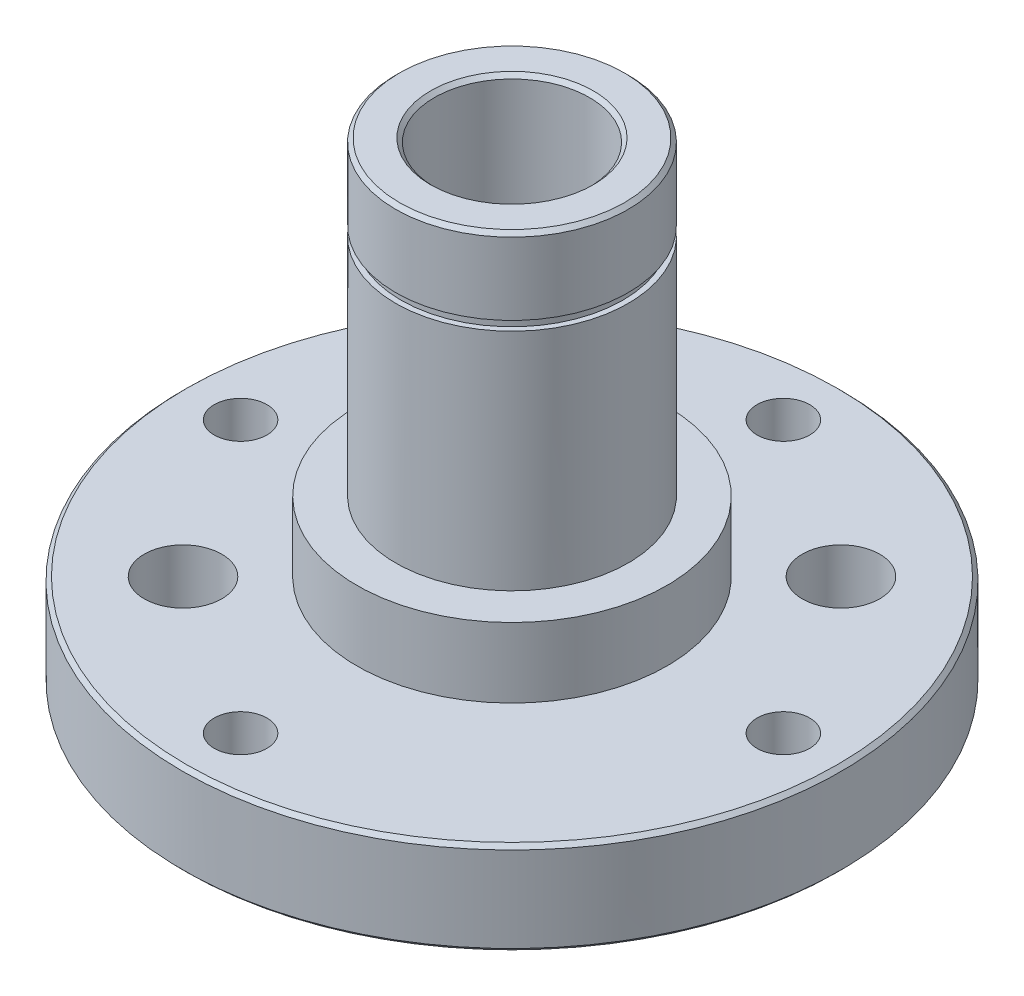
from build123d import *

# Parameters (mm, degrees)
SKETCH2_R                  = 10
CUT_EXTRUDE1_DEPTH         = 86.635856976
SKETCH3_W                  = 0.7
SKETCH3_H                  = 1.2
M8_TAPPED_HOLE1_D          = 6.8
F_10_0_10_DIAMETER_HOLE1_D = 10
CHAMFER1_SIZE              = 0.5


with BuildPart() as part:
    # Sketch1 → Revolve1 (revolve)
    with BuildSketch(Plane.XY, mode=Mode.PRIVATE) as revolve1_sk:
        Polygon((0, 0), (42.5, 0), (42.5, 12), (20, 12), (20, 21), (15, 21), (15, 61), (0, 61), align=None)
    revolve(revolve1_sk.sketch.rotate(Axis((0, 0, 0), (0, 1, 0)), 90), axis=Axis((0, 0, 0), (0, 1, 0)))

    # Sketch2 → Cut-Extrude1 (cut, through all)
    with BuildSketch(Plane(origin=(0, 61, 0), x_dir=(1, 0, 0), z_dir=(0, 1, 0))):
        with Locations(Location((0, 0, 0), (0, 0, 270))):
            Circle(SKETCH2_R)
    extrude(amount=-CUT_EXTRUDE1_DEPTH, mode=Mode.SUBTRACT)

    # Sketch3 → Cut-Revolve1 (revolve, cut)
    with BuildSketch(Plane.XY, mode=Mode.PRIVATE) as cut_revolve1_sk:
        with Locations((14.65, 50.6)):
            Rectangle(SKETCH3_W, SKETCH3_H)
    revolve(cut_revolve1_sk.sketch.rotate(Axis((0, 0, 0), (0, -1, 0)), 270), axis=Axis((0, 0, 0), (0, -1, 0)), mode=Mode.SUBTRACT)

    # M8 Tapped Hole1 (through all)
    with Locations(Plane(origin=(0, 12, 0), x_dir=(1, 0, 0), z_dir=(0, 1, 0))):
        with Locations((35, 0), (0, -35), (-35, 0), (0, 35), (0, 0)):
            Hole(M8_TAPPED_HOLE1_D / 2)

    # Ø10.0 (10) Diameter Hole1 (through all)
    with Locations(Plane(origin=(0, 12, 0), x_dir=(1, 0, 0), z_dir=(0, 1, 0))):
        with Locations((-21.213203436, -21.213203436), (21.213203436, 21.213203436)):
            Hole(F_10_0_10_DIAMETER_HOLE1_D / 2)

    # Chamfer1
    chamfer1_edges = [part.edges().sort_by_distance(p)[0] for p in [
        (0, 61, -10),
        (0, 61, 15),
        (0, 12, 42.5),
        (0, 0, 42.5),
    ]]
    chamfer(chamfer1_edges, length=CHAMFER1_SIZE)


solid = part.part
